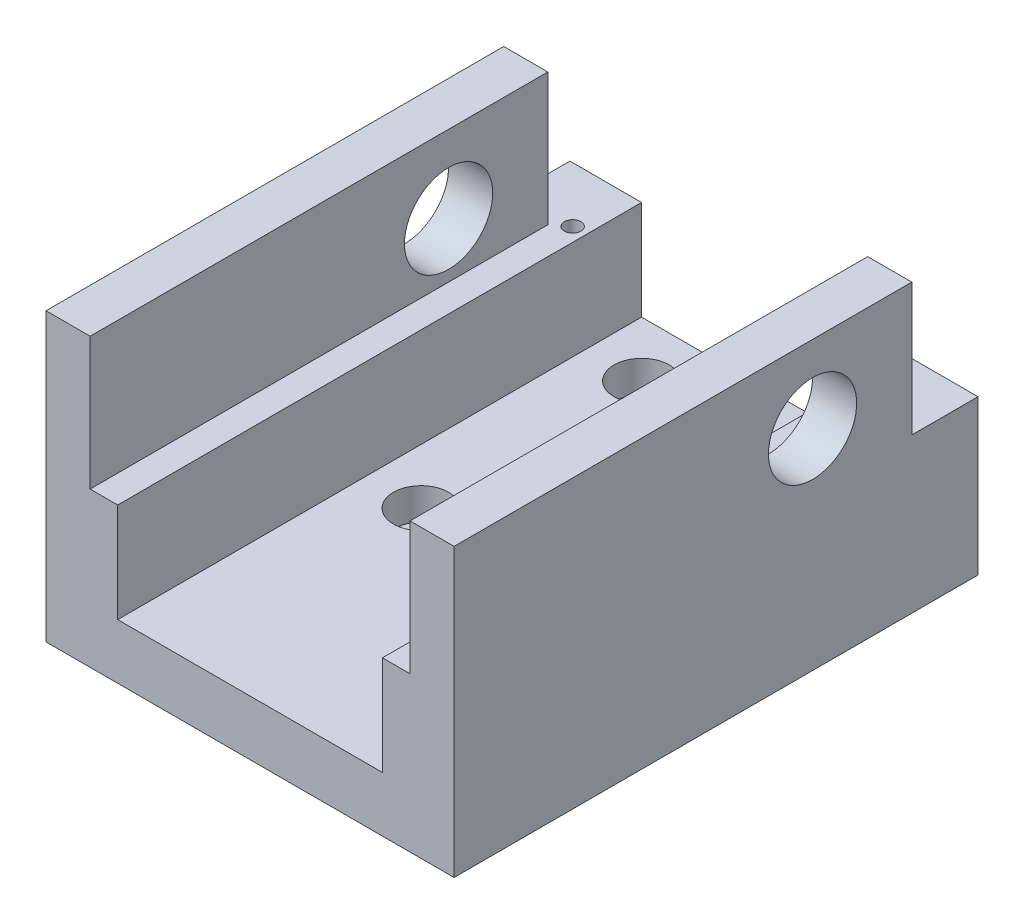
from build123d import *

# Parameters (mm, degrees)
EXTRUDE_1_DEPTH     = 95
SKETCH_2_R          = 2.75
CUT_EXTRUDE_1_DEPTH = 113.405897954
SKETCH_3_R          = 5
CUT_EXTRUDE_2_DEPTH = 5.75
SKETCH_4_W          = 12
SKETCH_4_H          = 24
CUT_EXTRUDE_3_DEPTH = 124.632519994
SKETCH_5_R          = 1.25
CUT_EXTRUDE_4_DEPTH = 7.5
SKETCH_6_R          = 1.5
CUT_EXTRUDE_5_DEPTH = 6
SKETCH_7_R          = 8
CUT_EXTRUDE_6_DEPTH = 124.632519994


with BuildPart() as part:
    # 草图1 → 凸台-拉伸1 (new body)
    with BuildSketch(Plane.XY):
        Polygon((-42.966101695, 24), (-42.966101695, -28), (31.033898305, -28), (31.033898305, 24), (23.033898305, 24), (23.033898305, 0), (18.033898305, 0), (18.033898305, -18), (-29.966101695, -18), (-29.966101695, 0), (-34.966101695, 0), (-34.966101695, 24), align=None)
    extrude(amount=EXTRUDE_1_DEPTH)

    # 草图2 → 切除-拉伸1 (cut, through all)
    with BuildSketch(Plane(origin=(0, -18, 0), x_dir=(1, 0, 0), z_dir=(0, 1, 0))):
        with Locations(Location((-19.966101695, -10, 0), (0, 0, 270))):
            Circle(SKETCH_2_R)
        with Locations(Location((-19.966101695, -50, 0), (0, 0, 270))):
            Circle(SKETCH_2_R)
        with Locations(Location((8.033898305, -10, 0), (0, 0, 270))):
            Circle(SKETCH_2_R)
        with Locations(Location((8.033898305, -50, 0), (0, 0, 270))):
            Circle(SKETCH_2_R)
    extrude(amount=-CUT_EXTRUDE_1_DEPTH, mode=Mode.SUBTRACT)

    # 草图3 → 切除-拉伸2 (cut)
    with BuildSketch(Plane(origin=(0, -18, 0), x_dir=(1, 0, 0), z_dir=(0, 1, 0))):
        with Locations(Location((-19.966101695, -10, 0), (0, 0, 270))):
            Circle(SKETCH_3_R)
        with Locations(Location((-19.966101695, -50, 0), (0, 0, 270))):
            Circle(SKETCH_3_R)
        with Locations(Location((8.033898305, -10, 0), (0, 0, 270))):
            Circle(SKETCH_3_R)
        with Locations(Location((8.033898305, -50, 0), (0, 0, 270))):
            Circle(SKETCH_3_R)
    extrude(amount=-CUT_EXTRUDE_2_DEPTH, mode=Mode.SUBTRACT)

    # 草图4 → 切除-拉伸3 (cut, through all)
    with BuildSketch(Plane.ZY.offset(42.966101695)):
        with Locations((6, 12)):
            Rectangle(SKETCH_4_W, SKETCH_4_H)
    extrude(amount=-CUT_EXTRUDE_3_DEPTH, mode=Mode.SUBTRACT)

    # 草图5 → 切除-拉伸4 (cut)
    with BuildSketch(Plane(origin=(0, 0, 0), x_dir=(1, 0, 0), z_dir=(0, 1, 0))):
        with Locations(Location((-32.466101695, -10, 0), (0, 0, 270))):
            Circle(SKETCH_5_R)
        with Locations(Location((20.533898305, -10, 0), (0, 0, 270))):
            Circle(SKETCH_5_R)
    extrude(amount=-CUT_EXTRUDE_4_DEPTH, mode=Mode.SUBTRACT)

    # 草图6 → 切除-拉伸5 (cut)
    with BuildSketch(Plane(origin=(0, 0, 0), x_dir=(1, 0, 0), z_dir=(0, 1, 0))):
        with Locations(Location((-32.466101695, -10, 0), (0, 0, 270))):
            Circle(SKETCH_6_R)
        with Locations(Location((20.533898305, -10, 0), (0, 0, 270))):
            Circle(SKETCH_6_R)
    extrude(amount=-CUT_EXTRUDE_5_DEPTH, mode=Mode.SUBTRACT)

    # 草图7 → 切除-拉伸6 (cut, through all)
    with BuildSketch(Plane.ZY.offset(42.966101695)):
        with Locations((30, 10)):
            Circle(SKETCH_7_R)
    extrude(amount=-CUT_EXTRUDE_6_DEPTH, mode=Mode.SUBTRACT)


solid = part.part
